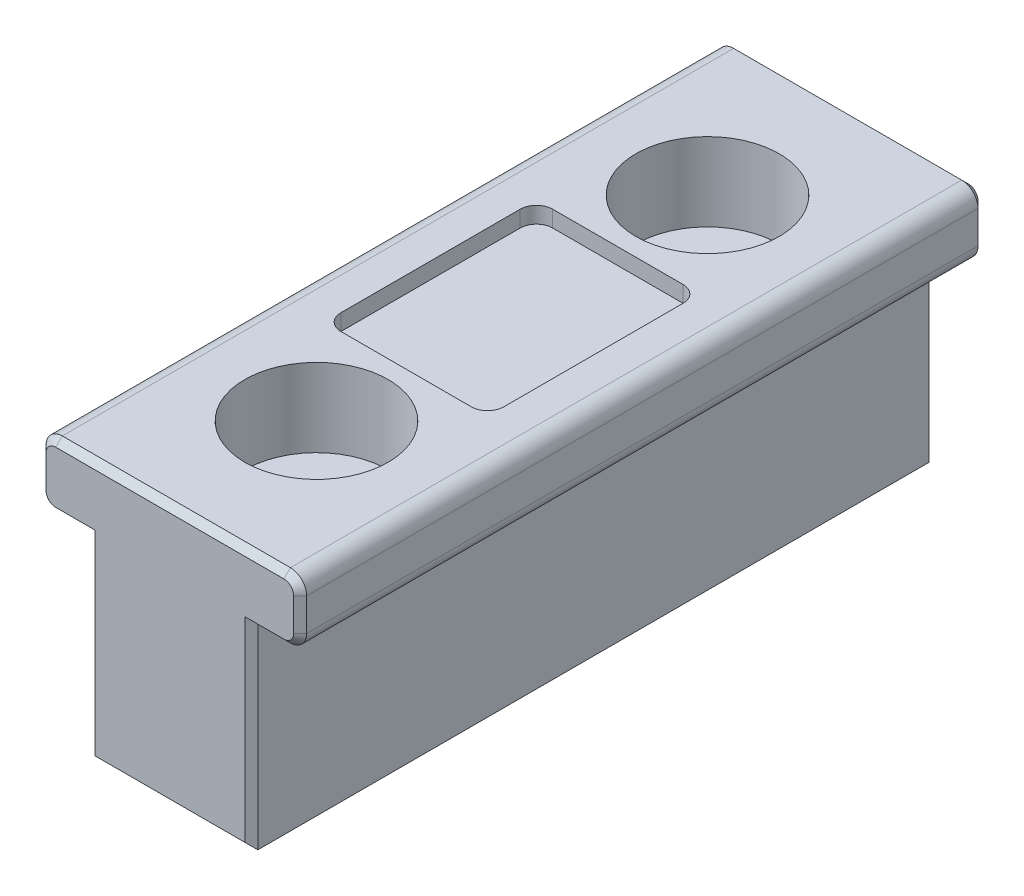
from build123d import *

# Parameters (mm, degrees)
SKETCH1_W                                           = 8
SKETCH1_H                                           = 8
BOSS_EXTRUDE1_DEPTH                                 = 21
SKETCH2_W                                           = 1.5
SKETCH2_H                                           = 6
CUT_EXTRUDE1_DEPTH                                  = 22.748563171
FILLET1_R                                           = 0.5
CBORE_FOR_M2_HEX_SOCKET_HEAD_CAP_SCREW1_D           = 2.4
CBORE_FOR_M2_HEX_SOCKET_HEAD_CAP_SCREW1_CBORE_D     = 4.4
CBORE_FOR_M2_HEX_SOCKET_HEAD_CAP_SCREW1_CBORE_DEPTH = 2.4
CHAMFER1_SIZE                                       = 0.2
SKETCH7_W                                           = 5
SKETCH7_H                                           = 6.5
CUT_EXTRUDE2_DEPTH                                  = 0.5
FILLET2_R                                           = 0.5


with BuildPart() as part:
    # Sketch1 → Boss-Extrude1 (new body)
    with BuildSketch(Plane.XY):
        Rectangle(SKETCH1_W, SKETCH1_H)
    extrude(amount=BOSS_EXTRUDE1_DEPTH)

    # Sketch2 → Cut-Extrude1 (cut, through all)
    with BuildSketch(Plane.XY.offset(21)):
        with Locations((-3.25, -1)):
            Rectangle(SKETCH2_W, SKETCH2_H)
        with Locations((3.25, -1)):
            Rectangle(SKETCH2_W, SKETCH2_H)
    extrude(amount=-CUT_EXTRUDE1_DEPTH, mode=Mode.SUBTRACT)

    # Fillet1
    fillet1_edges = [part.edges().sort_by_distance(p)[0] for p in [
        (-4, 2, 10.5),
        (4, 2, 10.5),
        (-4, 4, 10.5),
        (4, 4, 10.5),
    ]]
    fillet(fillet1_edges, radius=FILLET1_R)

    # CBORE for M2 Hex Socket Head Cap Screw1 (through all)
    with Locations(Plane(origin=(0, 4, 0), x_dir=(1, 0, 0), z_dir=(0, 1, 0))):
        with Locations((0, -4.5), (0, -16.5)):
            CounterBoreHole(CBORE_FOR_M2_HEX_SOCKET_HEAD_CAP_SCREW1_D / 2, CBORE_FOR_M2_HEX_SOCKET_HEAD_CAP_SCREW1_CBORE_D / 2, CBORE_FOR_M2_HEX_SOCKET_HEAD_CAP_SCREW1_CBORE_DEPTH)

    # Chamfer1
    chamfer1_edges = [part.edges().sort_by_distance(p)[0] for p in [
        (0, -4, 0),
        (0, -4, 21),
        (-3, 2, 0),
        (-2.5, -1, 0),
        (-2.5, -1, 21),
        (-3, 2, 21),
        (2.5, -1, 0),
        (2.5, -1, 21),
        (0, 4, 0),
        (0, 4, 21),
        (-4, 3, 0),
        (4, 3, 0),
        (3, 2, 0),
        (-3.853553391, 2.146446609, 0),
        (-3.853553391, 3.853553391, 0),
        (3.853553391, 2.146446609, 0),
        (3.853553391, 3.853553391, 0),
        (4, 3, 21),
        (3, 2, 21),
        (-4, 3, 21),
        (-3.853553391, 2.146446609, 21),
        (-3.853553391, 3.853553391, 21),
        (3.853553391, 2.146446609, 21),
        (3.853553391, 3.853553391, 21),
    ]]
    chamfer(chamfer1_edges, length=CHAMFER1_SIZE)

    # Sketch7 → Cut-Extrude2 (cut)
    with BuildSketch(Plane(origin=(0, 4, 0), x_dir=(1, 0, 0), z_dir=(0, 1, 0))):
        with Locations((0, -10.5)):
            Rectangle(SKETCH7_W, SKETCH7_H)
    extrude(amount=-CUT_EXTRUDE2_DEPTH, mode=Mode.SUBTRACT)

    # Fillet2
    fillet2_edges = [part.edges().sort_by_distance(p)[0] for p in [
        (2.5, 3.75, 7.25),
        (2.5, 3.75, 13.75),
        (-2.5, 3.75, 13.75),
        (-2.5, 3.75, 7.25),
    ]]
    fillet(fillet2_edges, radius=FILLET2_R)


solid = part.part
